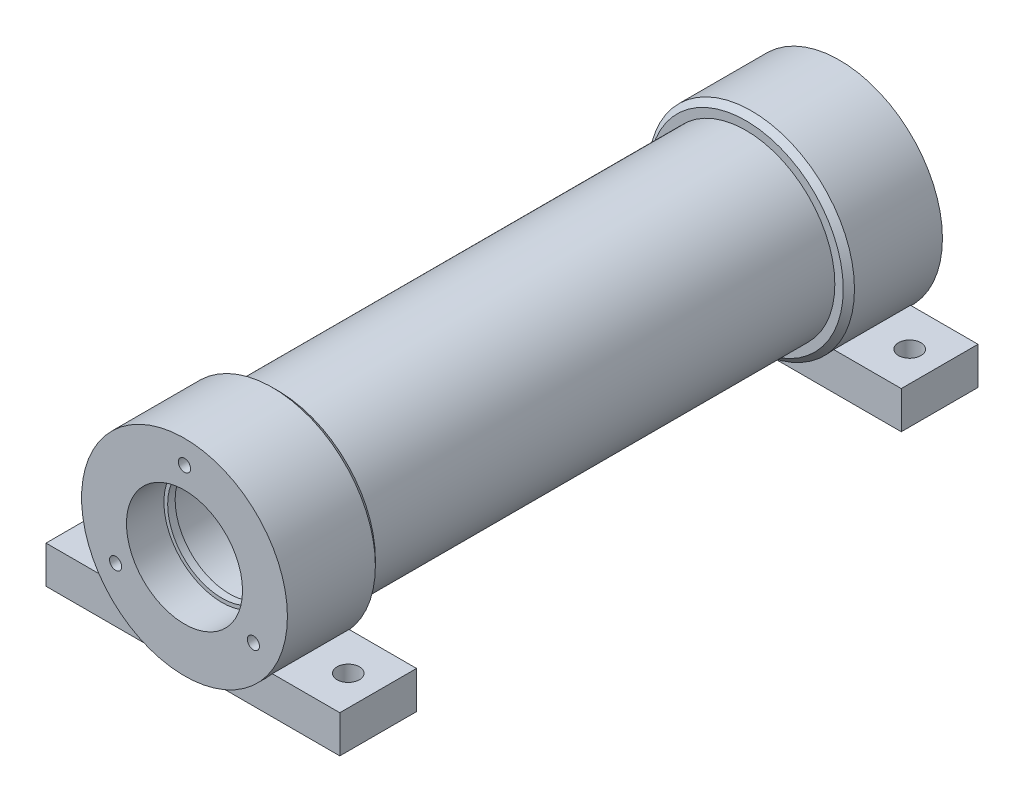
from build123d import *

# Parameters (mm, degrees)
SKETCH1_R           = 55
SKETCH1_R_2         = 29
BOSS_EXTRUDE1_DEPTH = 350
SKETCH3_W           = 157
SKETCH3_H           = 41
SKETCH3_R           = 6
BOSS_EXTRUDE2_DEPTH = 20
SKETCH6_R           = 31
SKETCH6_R_2         = 29
CUT_EXTRUDE1_DEPTH  = 344.638254564
CUT_EXTRUDE2_START  = -20
SKETCH8_R           = 31
CUT_EXTRUDE2_DEPTH  = 306
SKETCH9_R           = 36
CUT_EXTRUDE3_DEPTH  = 21
CUT_EXTRUDE4_DEPTH  = 5
SKETCH12_R          = 3.25
CUT_EXTRUDE5_DEPTH  = 5
CUT_EXTRUDE6_START  = -5
SKETCH13_R          = 3.25
CUT_EXTRUDE6_DEPTH  = 5
CUT_EXTRUDE7_START  = -300
SKETCH14_R          = 55
SKETCH14_R_2        = 47.5
CUT_EXTRUDE7_DEPTH  = 250
CHAMFER1_SIZE       = 3


with BuildPart() as part:
    # Sketch1 → Boss-Extrude1 (new body)
    with BuildSketch(Plane.XY):
        Circle(SKETCH1_R)
        Circle(SKETCH1_R_2, mode=Mode.SUBTRACT)
    extrude(amount=BOSS_EXTRUDE1_DEPTH)

    # Sketch3 → Boss-Extrude2 (add)
    # profile 1 of 2: a face of its own
    with BuildSketch(Plane(origin=(0, -55, 0), x_dir=(1, 0, 0), z_dir=(0, 1, 0))):
        with Locations((0, -25)):
            Rectangle(SKETCH3_W, SKETCH3_H)
        with Locations(Location((-62.5, -25, 0), (0, 0, 270))):
            Circle(SKETCH3_R, mode=Mode.SUBTRACT)
        with Locations(Location((62.5, -25, 0), (0, 0, 270))):
            Circle(SKETCH3_R, mode=Mode.SUBTRACT)
    # profile 2 of 2: a face of its own
    with BuildSketch(Plane(origin=(0, -55, 0), x_dir=(1, 0, 0), z_dir=(0, 1, 0))):
        with Locations((0, -325)):
            Rectangle(SKETCH3_W, SKETCH3_H)
        with Locations(Location((-62.5, -325, 0), (0, 0, 270))):
            Circle(SKETCH3_R, mode=Mode.SUBTRACT)
        with Locations(Location((62.5, -325, 0), (0, 0, 270))):
            Circle(SKETCH3_R, mode=Mode.SUBTRACT)
    extrude(amount=BOSS_EXTRUDE2_DEPTH)

    # Sketch6 → Cut-Extrude1 (cut, through all)
    with BuildSketch(Plane.XY.offset(330)):
        Circle(SKETCH6_R)
        Circle(SKETCH6_R_2, mode=Mode.SUBTRACT)
    extrude(amount=CUT_EXTRUDE1_DEPTH, mode=Mode.SUBTRACT)

    # Sketch8 → Cut-Extrude2 (cut)
    with BuildSketch(Plane(origin=(0, 0, 0), x_dir=(-1, 0, 0), z_dir=(0, 0, -1)).offset(CUT_EXTRUDE2_START)):
        with Locations(Location((0, 0, 0), (0, 0, 180))):
            Circle(SKETCH8_R)
    extrude(amount=-CUT_EXTRUDE2_DEPTH, mode=Mode.SUBTRACT)

    # Sketch9 → Cut-Extrude3 (cut)
    with BuildSketch(Plane(origin=(0, 0, 0), x_dir=(-1, 0, 0), z_dir=(0, 0, -1))):
        Circle(SKETCH9_R)
    extrude(amount=-CUT_EXTRUDE3_DEPTH, mode=Mode.SUBTRACT)

    # Sketch10 → Cut-Extrude4 (cut)
    with BuildSketch(Plane.XZ.offset(55)):
        with BuildLine():
            Line((-0.406572635, 14.221206443), (0.071479783, 14.311447227))
            Line((0.071479783, 14.311447227), (0.187823274, 14.336804141))
            Line((0.187823274, 14.336804141), (0.303420972, 14.371856347))
            Line((0.303420972, 14.371856347), (0.424239212, 14.417349635))
            Line((0.424239212, 14.417349635), (0.47420725, 14.437486008))
            Line((0.47420725, 14.437486008), (0.554752743, 14.477758754))
            Line((0.554752743, 14.477758754), (0.610687113, 14.427044925))
            Line((0.610687113, 14.427044925), (0.71136898, 14.3315836))
            add(Edge.make_bspline(
                [(0.71136898, 14.3315836), (0.721856091, 14.321145896), (0.740145648, 14.302942505), (0.760529505, 14.276154721), (0.773651987, 14.256318516), (0.776199491, 14.233996265), (0.753474145, 14.215550762), (0.73320985, 14.212558686), (0.721064271, 14.21076536)],
                knots=[0, 0, 0, 0, 1.501740704, 2.619040911, 3.421925612, 3.902833482, 4.743045209, 6, 6, 6, 6], degree=3))
            Line((0.721064271, 14.21076536), (0.222875479, 14.15035624))
            Line((0.222875479, 14.15035624), (-0.396131553, 14.060115456))
            Line((-0.396131553, 14.060115456), (-1.247079773, 13.928856134))
            Line((-1.247079773, 13.928856134), (-1.458884589, 13.893803928))
            Line((-1.458884589, 13.893803928), (-1.624450325, 13.858751723))
            Line((-1.624450325, 13.858751723), (-1.740793816, 13.833394808))
            Line((-1.740793816, 13.833394808), (-1.8310346, 13.813258435))
            Line((-1.8310346, 13.813258435), (-2.01226196, 13.752849315))
            add(Edge.make_bspline(
                [(-2.01226196, 13.752849315), (-2.016323505, 13.754435547), (-2.025739063, 13.758112784), (-2.040175334, 13.769142666), (-2.058685798, 13.783342977), (-2.071088478, 13.795919082), (-2.077891621, 13.802817352)],
                knots=[0, 0, 0, 0, 0.627088749, 1.453729905, 2.603314729, 4, 4, 4, 4], degree=3))
            Line((-2.077891621, 13.802817352), (-2.183794029, 13.903499219))
            add(Edge.make_bspline(
                [(-2.183794029, 13.903499219), (-2.190302659, 13.909664494), (-2.201789155, 13.920545034), (-2.2160876, 13.935204559), (-2.225114938, 13.946414269), (-2.229784962, 13.957426192), (-2.227110116, 13.968346688), (-2.225068312, 13.975876482), (-2.224066775, 13.979569963)],
                knots=[0, 0, 0, 0, 1.722921285, 3.040629084, 3.929144234, 4.488241117, 5.258458759, 6, 6, 6, 6], degree=3))
            Line((-2.224066775, 13.979569963), (-1.856391514, 14.019842709))
            Line((-1.856391514, 14.019842709), (-1.116566243, 14.124999326))
            Line((-1.116566243, 14.124999326), (-1.010663835, 14.135440408))
            Line((-1.010663835, 14.135440408), (-0.849572848, 14.160797323))
            Line((-0.849572848, 14.160797323), (-0.527390875, 14.21076536))
            add(Edge.make_bspline(
                [(-0.527390875, 14.21076536), (-0.5131185, 14.247021139), (-0.485789896, 14.316443349), (-0.44817178, 14.416731134), (-0.412707761, 14.507713345), (-0.381631609, 14.590094407), (-0.354247054, 14.663602778), (-0.328881613, 14.727522917), (-0.30956566, 14.783446495), (-0.286545434, 14.843602126), (-0.264611862, 14.909233157), (-0.240717815, 14.978954117), (-0.223714029, 15.039850248), (-0.21076841, 15.091089619), (-0.202459007, 15.133170956), (-0.194728394, 15.164868027), (-0.189803322, 15.187141612), (-0.186356826, 15.198453099), (-0.185072529, 15.202668194)],
                knots=[0, 0, 0, 0, 1.780201014, 3.408711381, 4.893688651, 6.241686147, 7.431484462, 8.477737141, 9.383124164, 10.134228723, 11.420168984, 12.544404274, 13.500791523, 14.307945422, 14.958445842, 15.459883076, 15.798731651, 16, 16, 16, 16], degree=3))
            Line((-0.185072529, 15.202668194), (-0.174631446, 15.338402266))
            Line((-0.174631446, 15.338402266), (-0.12988395, 15.363759181))
            Line((-0.12988395, 15.363759181), (0.036427578, 14.9356748))
            add(Edge.make_bspline(
                [(0.036427578, 14.9356748), (0.020626412, 14.921908661), (-0.00988882, 14.895323475), (-0.051310043, 14.85480513), (-0.086654203, 14.815495126), (-0.114176881, 14.782113622), (-0.136359131, 14.748596421), (-0.157515157, 14.710852564), (-0.185521238, 14.660984115), (-0.217415469, 14.597334445), (-0.257816877, 14.522225213), (-0.302085289, 14.433094624), (-0.352696528, 14.331492746), (-0.387979368, 14.25926752), (-0.406572635, 14.221206443)],
                knots=[0, 0, 0, 0, 0.889386884, 1.717585086, 2.457159812, 3.132776873, 3.551255267, 4.161138814, 4.968714737, 5.978618804, 7.18212222, 8.588306979, 10.202114145, 12, 12, 12, 12], degree=3))
        make_face()
        with BuildLine():
            Line((-1.569261747, 13.344901307), (-0.965170547, 13.47616063))
            Line((-0.965170547, 13.47616063), (-0.904761427, 13.617115243))
            add(Edge.make_bspline(
                [(-0.904761427, 13.617115243), (-0.901372718, 13.624236096), (-0.895205822, 13.63719488), (-0.886751347, 13.653724858), (-0.871967512, 13.658340322), (-0.858966977, 13.648084261), (-0.842765173, 13.633419382), (-0.83105625, 13.619832258), (-0.824215934, 13.611894702)],
                knots=[0, 0, 0, 0, 1.201991023, 2.187426594, 2.61300886, 3.330989457, 4.440772228, 6, 6, 6, 6], degree=3))
            Line((-0.824215934, 13.611894702), (-0.728754608, 13.491076462))
            add(Edge.make_bspline(
                [(-0.728754608, 13.491076462), (-0.723304678, 13.483506379), (-0.71355666, 13.469966152), (-0.703539054, 13.450253651), (-0.695894589, 13.435441116), (-0.692688102, 13.42030012), (-0.695423689, 13.403379114), (-0.700617604, 13.39152114), (-0.703397694, 13.385174054)],
                knots=[0, 0, 0, 0, 1.437865999, 2.571838831, 3.414042144, 4.001467023, 4.930267309, 6, 6, 6, 6], degree=3))
            Line((-0.703397694, 13.385174054), (-0.769027355, 13.304628561))
            add(Edge.make_bspline(
                [(-0.769027355, 13.304628561), (-0.774653084, 13.292123273), (-0.784881252, 13.269387342), (-0.792702738, 13.23858918), (-0.792830507, 13.211389583), (-0.793777748, 13.183322598), (-0.794603596, 13.146274272), (-0.794462867, 13.118677708), (-0.79438427, 13.103264827)],
                knots=[0, 0, 0, 0, 1.201973028, 2.185313705, 2.752348163, 3.580765237, 4.648839915, 6, 6, 6, 6], degree=3))
            Line((-0.79438427, 13.103264827), (-0.79438427, 11.522932417))
            add(Edge.make_bspline(
                [(-0.79438427, 11.522932417), (-0.794572018, 11.494840378), (-0.794989097, 11.432434486), (-0.797152873, 11.32999093), (-0.802258527, 11.209456588), (-0.806753137, 11.077663869), (-0.81278177, 10.947586774), (-0.821175539, 10.832993471), (-0.829157998, 10.739804554), (-0.8404754, 10.666938753), (-0.852407844, 10.611528579), (-0.861232133, 10.569424399), (-0.871273653, 10.540671757), (-0.882209618, 10.518753688), (-0.895486072, 10.50662704), (-0.910683562, 10.4951279), (-0.925406739, 10.506047), (-0.936476226, 10.525600711), (-0.955338224, 10.556596847), (-0.968138429, 10.581891409), (-0.975611629, 10.596659245)],
                knots=[0, 0, 0, 0, 1.299937258, 2.887784161, 4.741120287, 6.882270939, 8.989940936, 10.765980928, 12.199068736, 13.316796249, 14.174090439, 14.824211744, 15.300875456, 15.589150312, 15.93078443, 16.172629967, 16.332440572, 16.686813102, 17.233316318, 18, 18, 18, 18], degree=3))
            Line((-0.975611629, 10.596659245), (-1.050936581, 10.747309149))
            Line((-1.050936581, 10.747309149), (-1.161313739, 10.948672882))
            Line((-1.161313739, 10.948672882), (-1.378339096, 11.326043434))
            Line((-1.378339096, 11.326043434), (-1.34776164, 11.381977804))
            Line((-1.34776164, 11.381977804), (-1.071072955, 11.059795831))
            add(Edge.make_bspline(
                [(-1.071072955, 11.059795831), (-1.062464328, 11.049029316), (-1.046479246, 11.029037322), (-1.022882448, 11.002295608), (-1.003637618, 10.979319684), (-0.988322511, 10.960357208), (-0.97528142, 10.946837814), (-0.965895669, 10.937316798), (-0.960181528, 10.931983687), (-0.953124387, 10.929570792), (-0.952630243, 10.94331179), (-0.947552172, 10.955990772), (-0.944843147, 10.980894488), (-0.938446198, 11.022092472), (-0.931059956, 11.080545338), (-0.929968761, 11.143554003), (-0.930164345, 11.2034873), (-0.930100329, 11.266130613), (-0.930124534, 11.345931518), (-0.930120535, 11.404848856), (-0.930118342, 11.437166383)],
                knots=[0, 0, 0, 0, 1.090550141, 2.025007494, 2.820833353, 3.463036321, 3.950030695, 4.311650374, 4.508345549, 4.589445048, 4.819670847, 5.244277373, 5.861912751, 6.696419703, 8.597048854, 10.486244317, 11.686084884, 13.338324354, 15.442962726, 18, 18, 18, 18], degree=3))
            Line((-0.930118342, 11.437166383), (-0.930118342, 13.315069643))
            Line((-0.930118342, 13.315069643), (-1.543904832, 13.183810321))
            Line((-1.543904832, 13.183810321), (-1.543904832, 12.715453193))
            add(Edge.make_bspline(
                [(-1.543904832, 12.715453193), (-1.51876326, 12.720263929), (-1.470578849, 12.729483817), (-1.402248708, 12.745197088), (-1.340839688, 12.760901909), (-1.286718901, 12.776120328), (-1.240013732, 12.792039731), (-1.200334889, 12.807193478), (-1.167834301, 12.823491096), (-1.149526674, 12.835853858), (-1.141177366, 12.841491974)],
                knots=[0, 0, 0, 0, 1.447097256, 2.773395714, 3.963081848, 5.030690807, 5.950715991, 6.751962192, 7.430824462, 8, 8, 8, 8], degree=3))
            Line((-1.141177366, 12.841491974), (-1.020359126, 12.715453193))
            add(Edge.make_bspline(
                [(-1.020359126, 12.715453193), (-1.01300868, 12.706389838), (-1.001508506, 12.692209725), (-0.989223512, 12.667970012), (-1.002122816, 12.655211793), (-1.021300421, 12.651462499), (-1.04953642, 12.643782385), (-1.072727048, 12.641457656), (-1.085988787, 12.640128241)],
                knots=[0, 0, 0, 0, 1.421158395, 2.223479828, 2.61046817, 3.310932367, 4.462235937, 6, 6, 6, 6], degree=3))
            Line((-1.085988787, 12.640128241), (-1.206807027, 12.625212409))
            Line((-1.206807027, 12.625212409), (-1.543904832, 12.554362206))
            Line((-1.543904832, 12.554362206), (-1.543904832, 12.111361993))
            add(Edge.make_bspline(
                [(-1.543904832, 12.111361993), (-1.504525691, 12.119896898), (-1.429296625, 12.136201798), (-1.322683473, 12.166181438), (-1.227384168, 12.199057888), (-1.168865642, 12.225085639), (-1.141177366, 12.237400774)],
                knots=[0, 0, 0, 0, 1.142988193, 2.183540081, 3.14053467, 4, 4, 4, 4], degree=3))
            Line((-1.141177366, 12.237400774), (-1.030800208, 12.127023617))
            add(Edge.make_bspline(
                [(-1.030800208, 12.127023617), (-1.024221006, 12.120187035), (-1.012476237, 12.107982807), (-0.998416578, 12.09028614), (-0.991060274, 12.0751408), (-0.988854258, 12.061038375), (-0.998153504, 12.049314611), (-1.015247226, 12.042119694), (-1.040214653, 12.035751347), (-1.059845151, 12.032612046), (-1.071072955, 12.0308165)],
                knots=[0, 0, 0, 0, 1.354952739, 2.418774756, 3.196489366, 3.764968176, 4.325651609, 5.166302887, 6.379246607, 8, 8, 8, 8], degree=3))
            Line((-1.071072955, 12.0308165), (-1.206807027, 12.010680127))
            Line((-1.206807027, 12.010680127), (-1.322404726, 11.990543753))
            Line((-1.322404726, 11.990543753), (-1.543904832, 11.950271007))
            Line((-1.543904832, 11.950271007), (-1.543904832, 11.094848036))
            Line((-1.543904832, 11.094848036), (-1.549125373, 10.802497727))
            Line((-1.549125373, 10.802497727), (-1.559566456, 10.606354535))
            add(Edge.make_bspline(
                [(-1.559566456, 10.606354535), (-1.560705571, 10.590193284), (-1.562761491, 10.561024839), (-1.566890086, 10.521842963), (-1.575588333, 10.492164923), (-1.583543237, 10.471642323), (-1.59928627, 10.459001431), (-1.616816616, 10.471349501), (-1.631006668, 10.493206614), (-1.639486907, 10.513565653), (-1.644586699, 10.525809042)],
                knots=[0, 0, 0, 0, 1.653620154, 2.984517006, 4.012362575, 4.783820346, 5.26241329, 5.77288162, 6.660669754, 8, 8, 8, 8], degree=3))
            Line((-1.644586699, 10.525809042), (-1.690079987, 10.621270368))
            Line((-1.690079987, 10.621270368), (-1.740793816, 10.75252969))
            add(Edge.make_bspline(
                [(-1.740793816, 10.75252969), (-1.746018652, 10.764205722), (-1.754922028, 10.784102251), (-1.760670077, 10.812156127), (-1.753971886, 10.836029951), (-1.745620017, 10.863641531), (-1.733977513, 10.902657396), (-1.719534843, 10.943020037), (-1.707801674, 10.986764618), (-1.701253677, 11.034323691), (-1.694325743, 11.094709706), (-1.689727243, 11.168402877), (-1.685022576, 11.254897561), (-1.682239155, 11.354367685), (-1.680966981, 11.466745694), (-1.680585562, 11.546051568), (-1.680384696, 11.587816287)],
                knots=[0, 0, 0, 0, 0.636578029, 1.084760068, 1.375000506, 1.850988691, 2.521874947, 3.391460404, 3.977675852, 4.764263068, 5.769231626, 6.993061792, 8.425385581, 10.06616804, 11.928332685, 14, 14, 14, 14], degree=3))
            Line((-1.680384696, 11.587816287), (-1.680384696, 13.042855707))
            add(Edge.make_bspline(
                [(-1.680384696, 13.042855707), (-1.680585787, 13.076168213), (-1.68096698, 13.139316126), (-1.682222787, 13.228081221), (-1.684964222, 13.30568543), (-1.688458792, 13.353361138), (-1.690079987, 13.375478763)],
                knots=[0, 0, 0, 0, 1.201019177, 2.276678156, 3.200519768, 4, 4, 4, 4], degree=3))
            Line((-1.690079987, 13.375478763), (-1.71021636, 13.491076462))
            Line((-1.71021636, 13.491076462), (-1.730352733, 13.632031075))
            Line((-1.730352733, 13.632031075), (-1.680384696, 13.661862739))
            Line((-1.680384696, 13.661862739), (-1.569261747, 13.344901307))
        make_face()
        with BuildLine():
            Line((-1.398475469, 15.162395447), (-1.297793603, 15.046797749))
            Line((-1.297793603, 15.046797749), (-1.201586486, 14.9356748))
            Line((-1.201586486, 14.9356748), (-1.111345701, 14.825297642))
            Line((-1.111345701, 14.825297642), (-1.000222752, 14.688817779))
            add(Edge.make_bspline(
                [(-1.000222752, 14.688817779), (-0.991119605, 14.676490673), (-0.974843336, 14.654450021), (-0.955112595, 14.62375812), (-0.942078171, 14.599265771), (-0.935446432, 14.571816168), (-0.938499253, 14.534898767), (-0.942612733, 14.505034144), (-0.945034174, 14.487454045)],
                knots=[0, 0, 0, 0, 1.256855793, 2.247236429, 2.99537749, 3.519850422, 4.540036036, 6, 6, 6, 6], degree=3))
            Line((-0.945034174, 14.487454045), (-0.98530692, 14.286090312))
            add(Edge.make_bspline(
                [(-0.98530692, 14.286090312), (-0.988358416, 14.269947468), (-0.993642939, 14.241991604), (-1.002437563, 14.206209645), (-1.009748525, 14.184606661), (-1.020892228, 14.169403789), (-1.038841499, 14.177777988), (-1.043122648, 14.189032115), (-1.04571604, 14.195849528)],
                knots=[0, 0, 0, 0, 1.89514463, 3.28197485, 4.179259934, 4.624014091, 5.166468924, 6, 6, 6, 6], degree=3))
            Line((-1.04571604, 14.195849528), (-1.085988787, 14.311447227))
            Line((-1.085988787, 14.311447227), (-1.16653428, 14.532947333))
            Line((-1.16653428, 14.532947333), (-1.221722859, 14.668681405))
            Line((-1.221722859, 14.668681405), (-1.332845808, 14.895402053))
            Line((-1.332845808, 14.895402053), (-1.433527675, 15.107206869))
            Line((-1.433527675, 15.107206869), (-1.398475469, 15.162395447))
        make_face()
        with BuildLine():
            Line((-0.481897587, 13.47616063), (-0.441624841, 13.505992294))
            Line((-0.441624841, 13.505992294), (-0.225345275, 13.17411503))
            add(Edge.make_bspline(
                [(-0.225345275, 13.17411503), (-0.237751537, 13.153338608), (-0.262925692, 13.111180151), (-0.287750907, 13.040102552), (-0.303011379, 12.962967953), (-0.304909569, 12.909436064), (-0.305890769, 12.881764721)],
                knots=[0, 0, 0, 0, 0.942422429, 1.912315574, 2.92084823, 4, 4, 4, 4], degree=3))
            Line((-0.305890769, 12.881764721), (-0.305890769, 11.960712089))
            add(Edge.make_bspline(
                [(-0.305890769, 11.960712089), (-0.306049985, 11.928364378), (-0.306339216, 11.869601745), (-0.311228819, 11.790962857), (-0.316059167, 11.729118417), (-0.327407842, 11.687058119), (-0.335361874, 11.657327482), (-0.357984057, 11.646574128), (-0.377525389, 11.666960907), (-0.386116609, 11.683228355), (-0.391656803, 11.693718695)],
                knots=[0, 0, 0, 0, 2.030842012, 3.689213747, 4.962220867, 5.894200445, 6.467052584, 6.803517966, 7.228428264, 8, 8, 8, 8], degree=3))
            Line((-0.391656803, 11.693718695), (-0.43192955, 11.769043647))
            Line((-0.43192955, 11.769043647), (-0.472202296, 11.860030223))
            add(Edge.make_bspline(
                [(-0.472202296, 11.860030223), (-0.476294198, 11.871346487), (-0.483981369, 11.892605565), (-0.482561606, 11.915126775), (-0.481897587, 11.925659884)],
                knots=[0, 0, 0, 0, 1.064605406, 2, 2, 2, 2], degree=3))
            Line((-0.481897587, 11.925659884), (-0.456540673, 12.015900668))
            add(Edge.make_bspline(
                [(-0.456540673, 12.015900668), (-0.453078811, 12.027782561), (-0.444180799, 12.058322547), (-0.436698848, 12.112736539), (-0.427393729, 12.177961975), (-0.426938381, 12.224433023), (-0.426709009, 12.247841857)],
                knots=[0, 0, 0, 0, 0.632442273, 1.625564135, 2.803926823, 4, 4, 4, 4], degree=3))
            Line((-0.426709009, 12.247841857), (-0.43192955, 12.75572594))
            Line((-0.43192955, 12.75572594), (-0.43192955, 13.013024043))
            add(Edge.make_bspline(
                [(-0.43192955, 13.013024043), (-0.433436156, 13.037634103), (-0.436617084, 13.089593801), (-0.440582746, 13.158758084), (-0.446301567, 13.226180478), (-0.454831745, 13.294532531), (-0.466864942, 13.379795252), (-0.476586771, 13.442116135), (-0.481897587, 13.47616063)],
                knots=[0, 0, 0, 0, 0.95208706, 2.010159965, 2.675019936, 3.564457519, 4.669517981, 6, 6, 6, 6], degree=3))
        make_face()
        with BuildLine():
            Line((-0.436404299, 11.276075396), (-0.104527035, 11.003861461))
            add(Edge.make_bspline(
                [(-0.104527035, 11.003861461), (-0.089082477, 10.990731035), (-0.06229392, 10.967956338), (-0.025889872, 10.941440413), (-0.003907046, 10.92484366), (0.015835703, 10.918497304), (0.026215949, 10.931635614), (0.037016748, 10.941829031), (0.041855844, 10.958722539), (0.045320848, 10.980057666), (0.048210325, 11.010532911), (0.049397106, 11.060032673), (0.051043849, 11.118476905), (0.052996789, 11.174163645), (0.055559574, 11.218625656), (0.055745057, 11.263898), (0.056852625, 11.323055525), (0.056666449, 11.367309437), (0.056563951, 11.391673095)],
                knots=[0, 0, 0, 0, 1.553735856, 2.69495192, 3.412699307, 3.722326834, 4.114439698, 4.533317644, 4.876210397, 5.417202451, 6.20073591, 7.209527591, 9.20747069, 10.673142458, 11.472898917, 12.614273472, 14.136013762, 16, 16, 16, 16], degree=3))
            Line((0.056563951, 11.391673095), (0.056563951, 13.093569536))
            add(Edge.make_bspline(
                [(0.056563951, 13.093569536), (0.056233411, 13.140801342), (0.055627998, 13.227310366), (0.055927331, 13.345428183), (0.052371014, 13.439877013), (0.049660615, 13.513738259), (0.045859135, 13.572180586), (0.041130343, 13.620613826), (0.037175116, 13.661746525), (0.033063439, 13.686489432), (0.031207037, 13.697660736)],
                knots=[0, 0, 0, 0, 1.873185307, 3.430896396, 4.683576418, 5.620985941, 6.362032253, 7.00557425, 7.551021544, 8, 8, 8, 8], degree=3))
            Line((0.031207037, 13.697660736), (-0.003845169, 13.883362846))
            Line((-0.003845169, 13.883362846), (0.036427578, 13.939297216))
            Line((0.036427578, 13.939297216), (0.283284599, 13.59697887))
            add(Edge.make_bspline(
                [(0.283284599, 13.59697887), (0.272728495, 13.574161823), (0.253236038, 13.532028828), (0.228096918, 13.473443207), (0.211136936, 13.423870938), (0.200943231, 13.379608287), (0.196902442, 13.332785011), (0.193982835, 13.275833515), (0.192881665, 13.204445387), (0.192503898, 13.151988899), (0.192298023, 13.123401201)],
                knots=[0, 0, 0, 0, 1.233182776, 2.277143302, 3.125453663, 3.799970514, 4.498845952, 5.426842513, 6.597682513, 8, 8, 8, 8], degree=3))
            Line((0.192298023, 13.123401201), (0.192298023, 11.084406954))
            add(Edge.make_bspline(
                [(0.192298023, 11.084406954), (0.19196125, 11.05680784), (0.191263173, 10.999599186), (0.187161164, 10.914847847), (0.183358045, 10.834998274), (0.179239221, 10.78483969), (0.177382191, 10.762224981)],
                knots=[0, 0, 0, 0, 1.026628304, 2.12804016, 3.156000343, 4, 4, 4, 4], degree=3))
            Line((0.177382191, 10.762224981), (0.162466359, 10.611575077))
            add(Edge.make_bspline(
                [(0.162466359, 10.611575077), (0.160148635, 10.588640118), (0.156152888, 10.549100343), (0.146317558, 10.499405596), (0.14026351, 10.466878167), (0.124638969, 10.447270941), (0.107223007, 10.448469506), (0.091646973, 10.448141577), (0.08285717, 10.461096499), (0.070611571, 10.47662461), (0.05559864, 10.50380895), (0.043438358, 10.524386518), (0.036427578, 10.536250125)],
                knots=[0, 0, 0, 0, 2.275990337, 3.923798011, 5.003779201, 5.542511237, 6.185414382, 6.633666531, 6.964142247, 7.632357099, 8.634980329, 10, 10, 10, 10], degree=3))
            Line((0.036427578, 10.536250125), (-0.038897374, 10.651847823))
            Line((-0.038897374, 10.651847823), (-0.150020323, 10.807718269))
            Line((-0.150020323, 10.807718269), (-0.366299889, 11.084406954))
            Line((-0.366299889, 11.084406954), (-0.461761214, 11.215666276))
            Line((-0.461761214, 11.215666276), (-0.436404299, 11.276075396))
        make_face()
    extrude(amount=-CUT_EXTRUDE4_DEPTH, mode=Mode.SUBTRACT)

    # Sketch12 → Cut-Extrude5 (cut)
    with BuildSketch(Plane(origin=(0, 0, 0), x_dir=(-1, 0, 0), z_dir=(0, 0, -1))):
        with Locations((0, 42.5)):
            Circle(SKETCH12_R)
        with Locations((-36.806079661, -21.25)):
            Circle(SKETCH12_R)
        with Locations((36.806079661, -21.25)):
            Circle(SKETCH12_R)
    extrude(amount=-CUT_EXTRUDE5_DEPTH, mode=Mode.SUBTRACT)

    # Sketch13 → Cut-Extrude6 (cut)
    with BuildSketch(Plane.XY.offset(350).offset(CUT_EXTRUDE6_START)):
        with Locations(Location((0, 42.5, 0), (0, 0, 180))):
            Circle(SKETCH13_R)
        with Locations(Location((-36.806079661, -21.25, 0), (0, 0, 180))):
            Circle(SKETCH13_R)
        with Locations(Location((36.806079661, -21.25, 0), (0, 0, 180))):
            Circle(SKETCH13_R)
    extrude(amount=CUT_EXTRUDE6_DEPTH, mode=Mode.SUBTRACT)

    # Sketch14 → Cut-Extrude7 (cut)
    with BuildSketch(Plane.XY.offset(350).offset(CUT_EXTRUDE7_START)):
        Circle(SKETCH14_R)
        Circle(SKETCH14_R_2, mode=Mode.SUBTRACT)
    extrude(amount=CUT_EXTRUDE7_DEPTH, mode=Mode.SUBTRACT)

    # Chamfer1
    chamfer1_edges = [part.edges().sort_by_distance(p)[0] for p in [
        (-55, 0, 50),
        (-55, 0, 300),
    ]]
    chamfer(chamfer1_edges, length=CHAMFER1_SIZE)


solid = part.part
